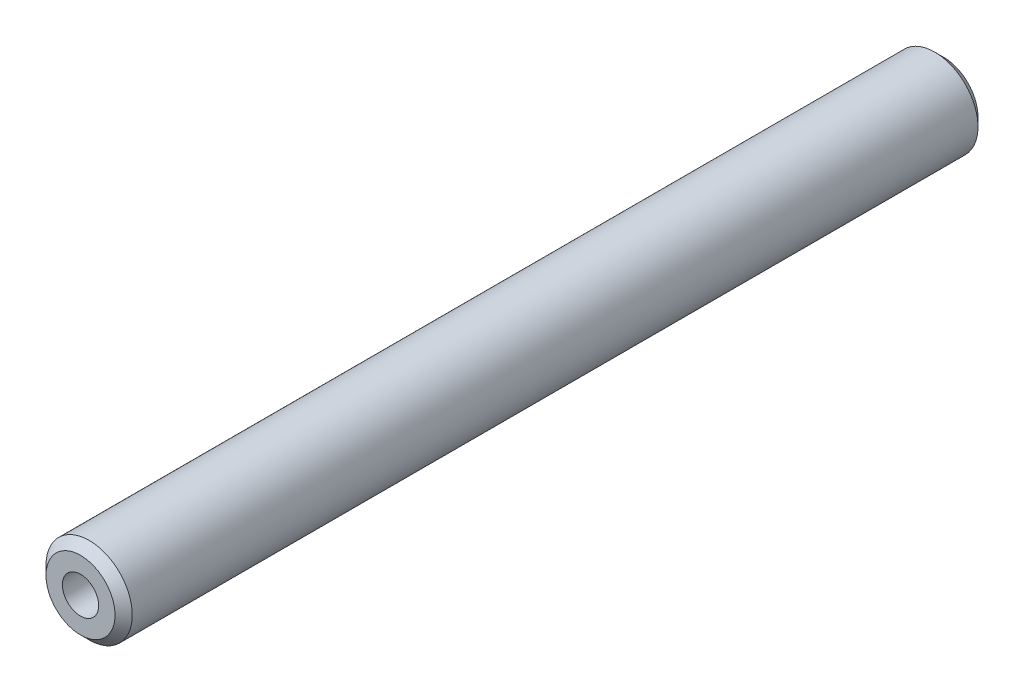
from build123d import *


with BuildPart() as part:
    # 草图1 → 旋转1 (revolve)
    with BuildSketch(Plane.XZ, mode=Mode.PRIVATE) as revolve_1_sk:
        Polygon((2.1, 37.6), (0, 36.3381927), (0, -36.3381927), (2.1, -37.6), (2.1, -50), (4, -50), (5, -49), (5, 49), (4, 50), (2.1, 50), align=None)
    revolve(revolve_1_sk.sketch.rotate(Axis((0, 0, 50), (0, 0, -1)), 180), axis=Axis((0, 0, 50), (0, 0, -1)))


solid = part.part
